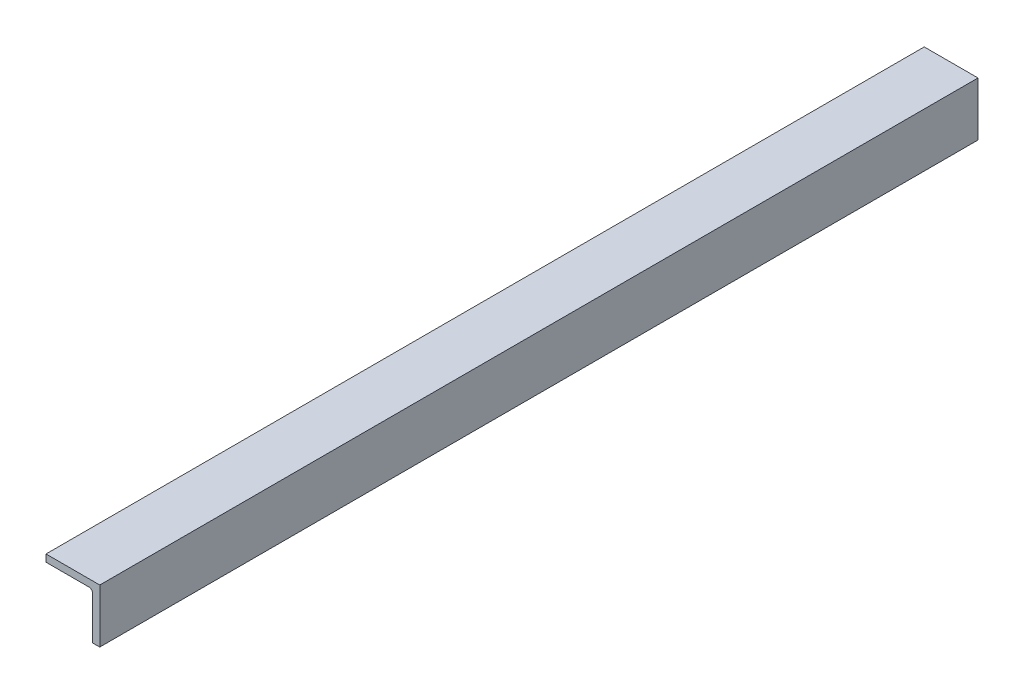
from build123d import *

# Parameters (mm, degrees)
BOSS_EXTRUDE1_DEPTH = 490


with BuildPart() as part:
    # Sketch1 → Boss-Extrude1 (new body)
    with BuildSketch(Plane.XY):
        with BuildLine():
            Line((0, 0), (30, 0))
            Line((30, 0), (30, -30))
            Line((30, -30), (26, -30))
            Line((26, -30), (26, -6))
            ThreePointArc((26, -6), (25.414213562, -4.585786438), (24, -4))
            Line((24, -4), (0, -4))
            Line((0, -4), (0, 0))
        make_face()
    extrude(amount=BOSS_EXTRUDE1_DEPTH)


solid = part.part
